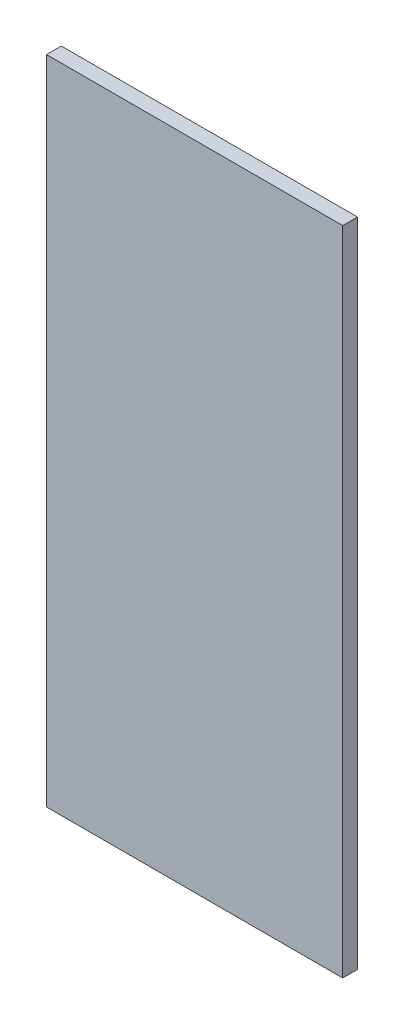
SolidWorks part; units mm, degrees
ref_plane "前视基准面" through (0, 0, 0) normal (0, 0, 1) x (1, 0, 0)
ref_plane "上视基准面" through (0, 0, 0) normal (0, 1, 0) x (1, 0, 0)
ref_plane "右视基准面" through (0, 0, 0) normal (1, 0, 0) x (0, 0, -1)
sketch "草图1" plane through (0, 0, 0) normal (0, 0, 1) x (1, 0, 0)
  line L1 (-50, 110) -> (50, 110)
  line L2 (-50, 110) -> (-50, -110)
  line L3 (-50, -110) -> (50, -110)
  line L4 (50, 110) -> (50, -110)
  line L5 (-50, 110) -> (50, -110) construction
  line L6 (-50, -110) -> (50, 110) construction
  point P0 (0, 0)
  dimension "D1" = 220
  dimension "D2" = 100
extrude "凸台-拉伸1" add sketch "草图1" along normal blind 5
